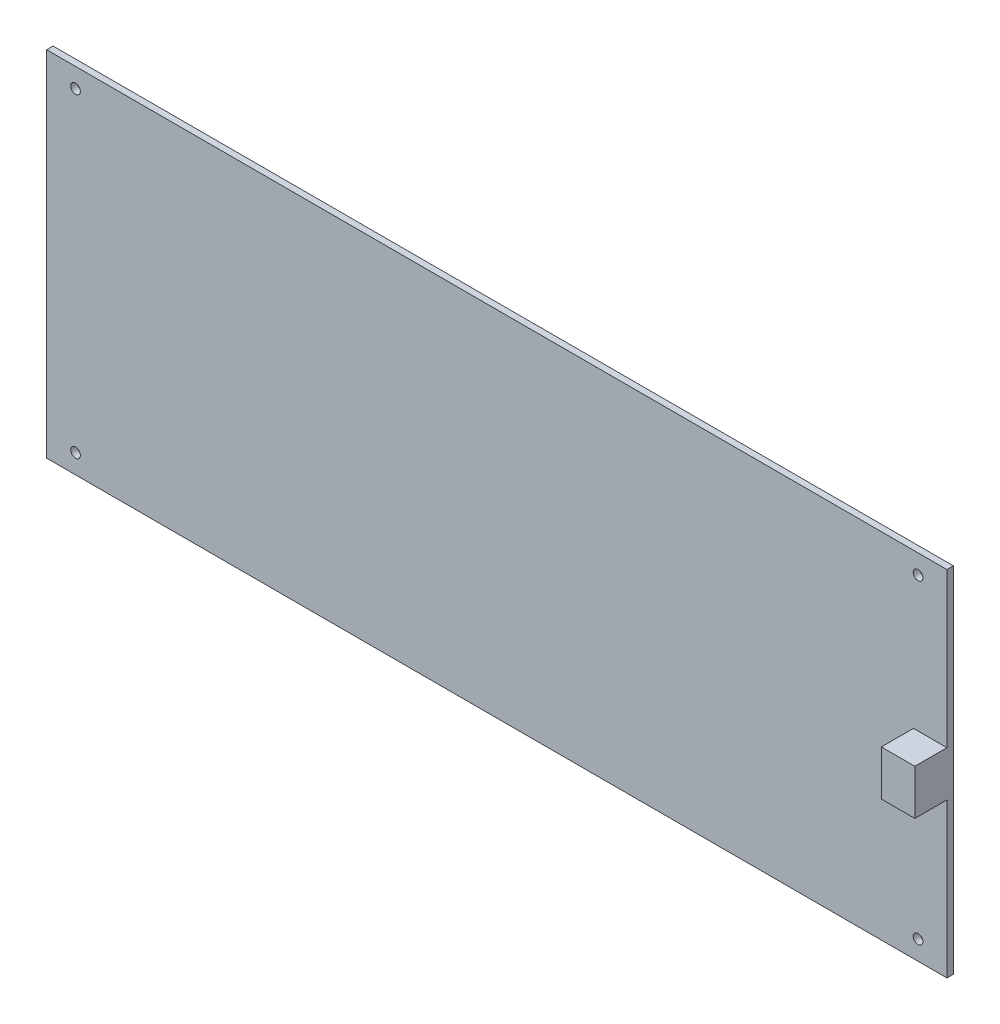
from build123d import *

# Parameters (mm, degrees)
SKETCH1_W           = 140
SKETCH1_H           = 55
SKETCH1_R           = 0.75
BOSS_EXTRUDE1_DEPTH = 1
SKETCH2_W           = 5.209314299
SKETCH2_H           = 7.02492173
BOSS_EXTRUDE2_DEPTH = 5


with BuildPart() as part:
    # Sketch1 → Boss-Extrude1 (new body)
    with BuildSketch(Plane.XY):
        Rectangle(SKETCH1_W, SKETCH1_H)
        with Locations((-65.5, -24.5)):
            Circle(SKETCH1_R, mode=Mode.SUBTRACT)
        with Locations((-65.5, 24.5)):
            Circle(SKETCH1_R, mode=Mode.SUBTRACT)
        with Locations((65.5, 24.5)):
            Circle(SKETCH1_R, mode=Mode.SUBTRACT)
        with Locations((65.5, -24.5)):
            Circle(SKETCH1_R, mode=Mode.SUBTRACT)
    extrude(amount=BOSS_EXTRUDE1_DEPTH)

    # Sketch2 → Boss-Extrude2 (add)
    with BuildSketch(Plane.XY.offset(1)):
        with Locations((67.395342851, 0)):
            Rectangle(SKETCH2_W, SKETCH2_H)
    extrude(amount=BOSS_EXTRUDE2_DEPTH)


solid = part.part
